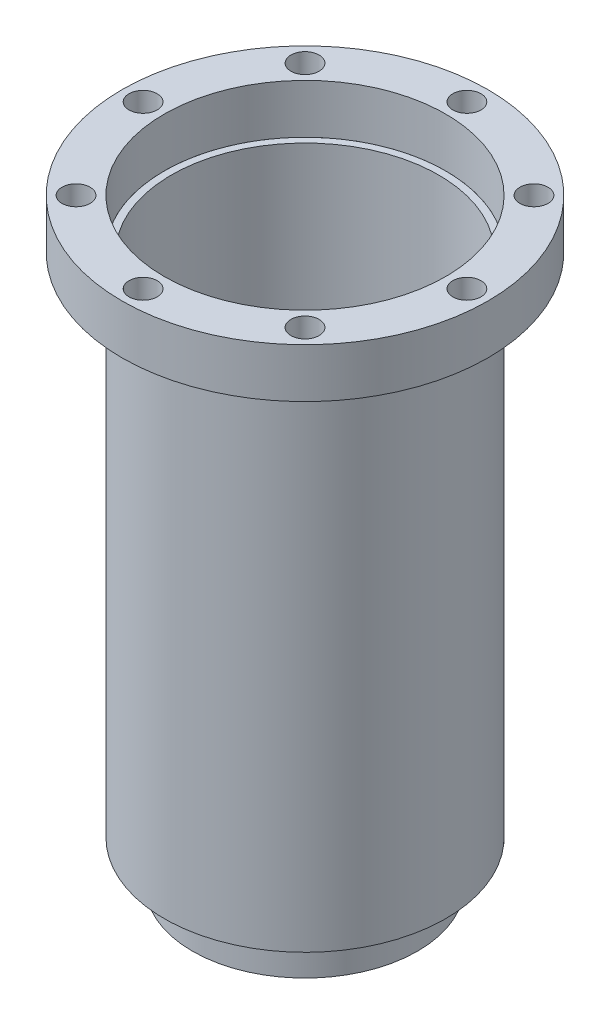
SolidWorks part; units mm, degrees
ref_plane "Front Plane" through (0, 0, 0) normal (0, 0, 1) x (1, 0, 0)
ref_plane "Top Plane" through (0, 0, 0) normal (0, 1, 0) x (1, 0, 0)
ref_plane "Right Plane" through (0, 0, 0) normal (1, 0, 0) x (0, 0, -1)
other "Configuration Table"
sketch "Sketch1" plane through (0, 0, 0) normal (0, 1, 0) x (1, 0, 0)
  circle A0 centre (0, 0) radius 100
extrude "Boss-Extrude1" add sketch "Sketch1" along normal blind 360
shell "Shell1" thickness 10
sketch "Sketch2" plane through (0, 10, 0) normal (0, 1, 0) x (1, 0, 0)
  circle A0 centre (0, 0) radius 70
  circle A1 centre (0, 0) radius 100 construction
  dimension "D1" = 30
extrude "Cut-Extrude1" cut sketch "Sketch2" against normal blind 300
sketch "Sketch3" plane through (0, 0, 0) normal (0, -1, 0) x (1, 0, 0)
  circle A0 centre (0, 0) radius 70
  circle A1 centre (0, 0) radius 80
  dimension "D1" = 140
  dimension "D2" = 10
extrude "Boss-Extrude2" add sketch "Sketch3" along normal blind 30
sketch "Sketch4" plane through (0, 360, 0) normal (0, 1, 0) x (1, 0, 0)
  circle A0 centre (0, 0) radius 130
  circle A1 centre (0, 0) radius 100
  dimension "D1" = 200
  dimension "D2" = 30
extrude "Boss-Extrude3" add sketch "Sketch4" along normal blind 35
sketch "Sketch6" plane through (0, 360, 0) normal (0, 1, 0) x (1, 0, 0)
  circle A0 centre (0, 0) radius 95
  circle A1 centre (0, 0) radius 90 construction
  circle A2 centre (0, 0) radius 90
  dimension "D1" = 5
extrude "Cut-Extrude3" cut sketch "Sketch6" against normal up to surface (309 mm away) and the other way through all
sketch "Sketch7" plane through (0, 395, 0) normal (0, 1, 0) x (1, 0, 0)
  circle A0 centre (-115, 0) radius 10
  dimension "D1" = 20
  dimension "D2" = 115
extrude "Cut-Extrude6" cut sketch "Sketch7" against normal through all both and the other way through all
pattern_circular "CirPattern1" count 8 over 360 about axis through (0, 0, 0) along (0, 1, 0) of "Cut-Extrude6"
sketch "Sketch8" plane through (0, 395, 0) normal (0, 1, 0) x (1, 0, 0)
  circle A0 centre (0, 0) radius 25.082
